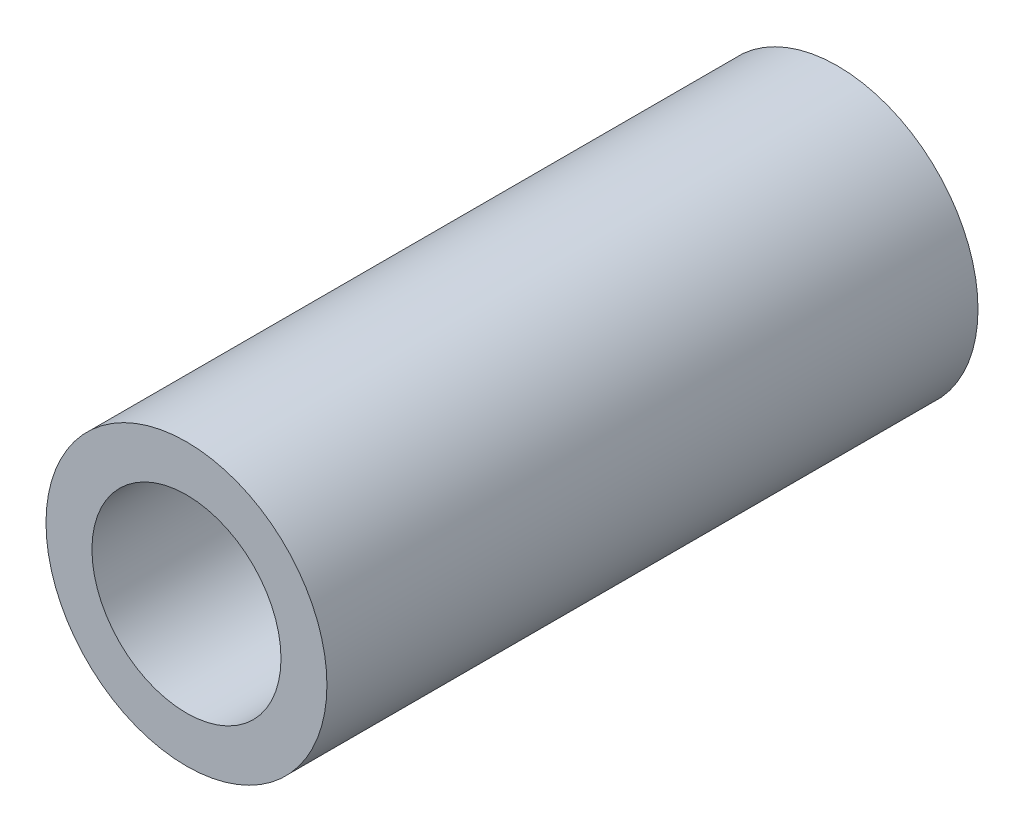
SolidWorks part; units mm, degrees
material "普通碳钢"
ref_plane "Front Plane" through (0, 0, 0) normal (0, 0, 1) x (1, 0, 0)
ref_plane "Top Plane" through (0, 0, 0) normal (0, 1, 0) x (1, 0, 0)
ref_plane "Right Plane" through (0, 0, 0) normal (1, 0, 0) x (0, 0, -1)
sketch "Sketch1" plane through (0, 0, 0) normal (0, 0, 1) x (1, 0, 0)
  circle A0 centre (0, 0) radius 6.85
  circle A1 centre (0, 0) radius 4.61
  dimension "D1" = 13.7
  dimension "D2" = 2.24
extrude "Boss-Extrude1" add sketch "Sketch1" along normal mid plane 31.75
